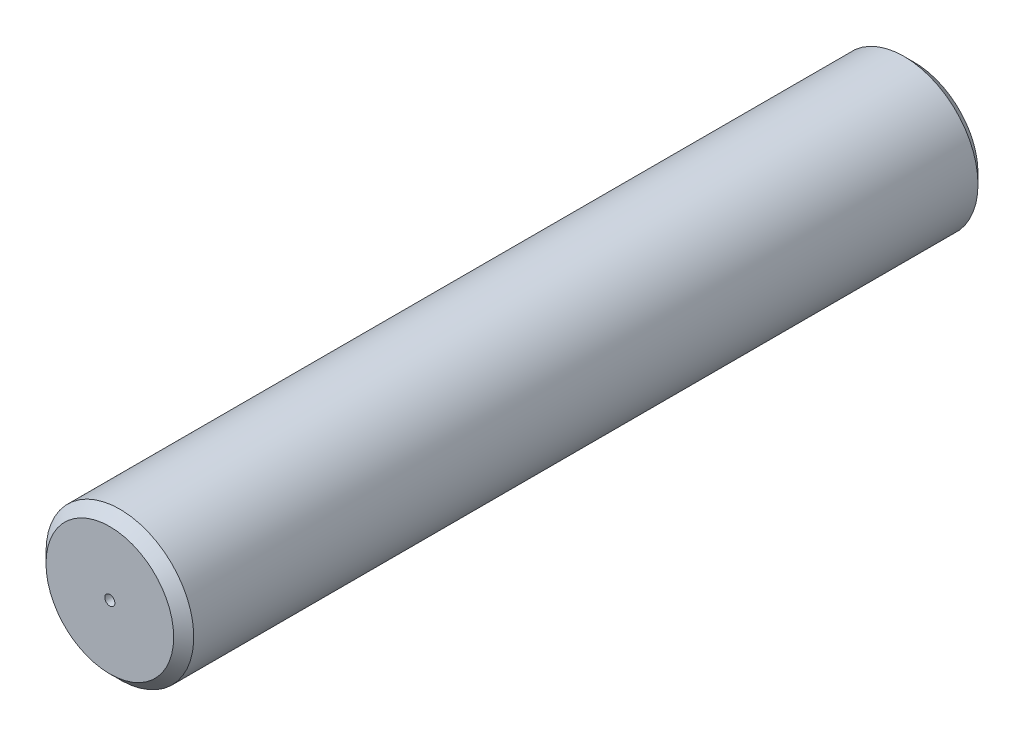
SolidWorks part; units mm, degrees
ref_plane "Front Plane" through (0, 0, 0) normal (0, 0, 1) x (1, 0, 0)
ref_plane "Top Plane" through (0, 0, 0) normal (0, 1, 0) x (1, 0, 0)
ref_plane "Right Plane" through (0, 0, 0) normal (1, 0, 0) x (0, 0, -1)
other "Configuration Table"
sketch "Sketch1" plane through (0, 0, 0) normal (0, 0, 1) x (1, 0, 0)
  circle A1 centre (-27.0657, 0) radius 3.6746
extrude "Boss-Extrude1" add sketch "Sketch1" along normal mid plane 40
chamfer "Chamfer2" distance 0.5 angle 45 2 edges at (-23.3911, 0, -20) (-23.3911, 0, 20)
sketch "Sketch2" plane through (0, 0, 20) normal (0, 0, 1) x (1, 0, 0)
  circle A0 centre (-27.0657, 0) radius 0.25
extrude "Cut-Extrude1" cut sketch "Sketch2" against normal blind 1 draft 3
mirror "Mirror1" about plane through (0, 0, 0) normal (0, 0, 1) of "Cut-Extrude1"
